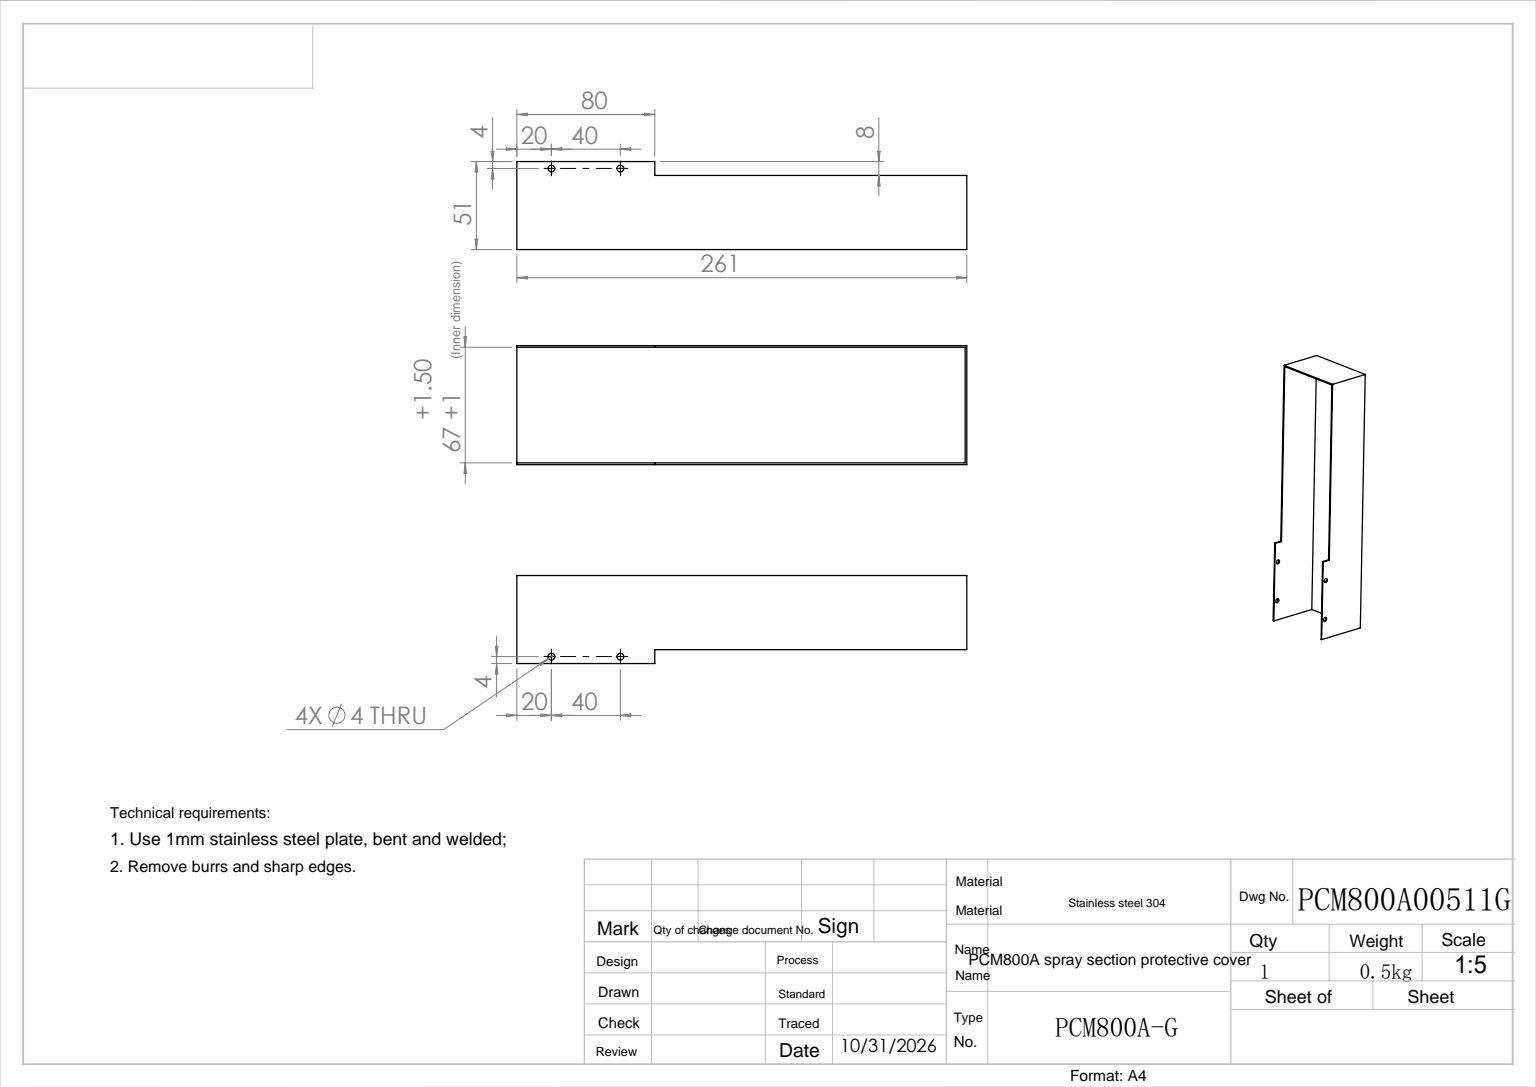
from build123d import *

# Parameters (mm, degrees)
EXTRUDE_1_DEPTH        = 67
SHELL_1_T              = 1
SKETCH_2_R             = 2
CUT_EXTRUDE_1_DEPTH    = 404.809707905
PATTERN_LINEAR_1_COUNT = 2
PATTERN_LINEAR_1_PITCH = 40


with BuildPart() as part:
    # 草图1 → 凸台-拉伸1 (new body)
    with BuildSketch(Plane.XY):
        Polygon((5.123141908, -134.949925194), (5.123141908, -314.949925194), (-2.876858092, -314.949925194), (-2.876858092, -394.949925194), (47.123141908, -394.949925194), (47.123141908, -134.949925194), align=None)
    extrude(amount=EXTRUDE_1_DEPTH)

    # 抽壳1
    shell_1_openings = [part.faces().sort_by_distance(p)[0] for p in [
        (5.123141908, -224.949925194, 33.5),
        (1.123141908, -314.949925194, 33.5),
        (-2.876858092, -354.949925194, 33.5),
        (22.123141908, -394.949925194, 33.5),
    ]]
    offset(amount=SHELL_1_T, openings=shell_1_openings, kind=Kind.INTERSECTION)

    # 草图2 → 切除-拉伸1 (cut, through all)
    with BuildSketch(Plane.XY.offset(68)):
        with Locations((1.123141908, -374.949925194)):
            Circle(SKETCH_2_R)
    cut_extrude_1 = extrude(amount=-CUT_EXTRUDE_1_DEPTH, mode=Mode.SUBTRACT)

    # 阵列(线性)1: 切除-拉伸1 ×2
    with Locations(*[(0, i * PATTERN_LINEAR_1_PITCH, 0) for i in range(1, PATTERN_LINEAR_1_COUNT)]):
        add(cut_extrude_1, mode=Mode.SUBTRACT)


solid = part.part
